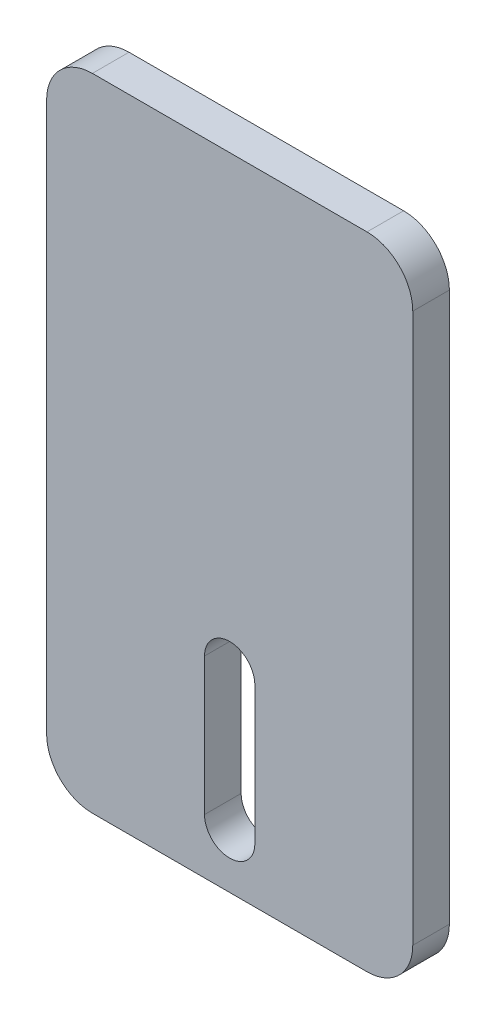
SolidWorks part; units mm, degrees
material "Q235"
ref_plane "Front Plane" through (0, 0, 0) normal (0, 0, 1) x (1, 0, 0)
ref_plane "Top Plane" through (0, 0, 0) normal (0, 1, 0) x (1, 0, 0)
ref_plane "Right Plane" through (0, 0, 0) normal (1, 0, 0) x (0, 0, -1)
sketch "Sketch1" plane through (0, 0, 0) normal (0, 0, 1) x (1, 0, 0)
  line L1 (10, 0) -> (70, 0)
  line L2 (0, 10) -> (0, 130)
  line L3 (10, 140) -> (70, 140)
  line L4 (80, 10) -> (80, 130)
  arc A2 (80, 10) -> (70, 0) centre (70, 10) cw
  arc A3 (10, 0) -> (0, 10) centre (10, 10) cw
  arc A4 (80, 130) -> (70, 140) centre (70, 130) ccw
  arc A5 (0, 130) -> (10, 140) centre (10, 130) cw
  point P14 (80, 0)
  point P17 (0, 0)
  point P22 (0, 140)
  dimension "D7" = 10
  dimension "D1" = 80
  dimension "D2" = 140
extrude "Boss-Extrude1" add sketch "Sketch1" along normal blind 8
sketch "Sketch2" plane through (0, 0, 8) normal (0, 0, 1) x (1, 0, 0)
  line L0 (40, 12) -> (40, 42) construction
  line L1 (34.5, 12) -> (34.5, 42)
  line L2 (45.5, 12) -> (45.5, 42)
  line L3 (10, 0) -> (70, 0) construction
  line L4 (40, 0) -> (40, 12) construction
  arc A0 (34.5, 12) -> (45.5, 12) centre (40, 12) ccw
  arc A1 (45.5, 42) -> (34.5, 42) centre (40, 42) ccw
  point P2 (40, 27)
  dimension "D2" = 12
  dimension "D1" = 11
  dimension "D3" = 30
extrude "Cut-Extrude1" cut sketch "Sketch2" against normal blind 10
